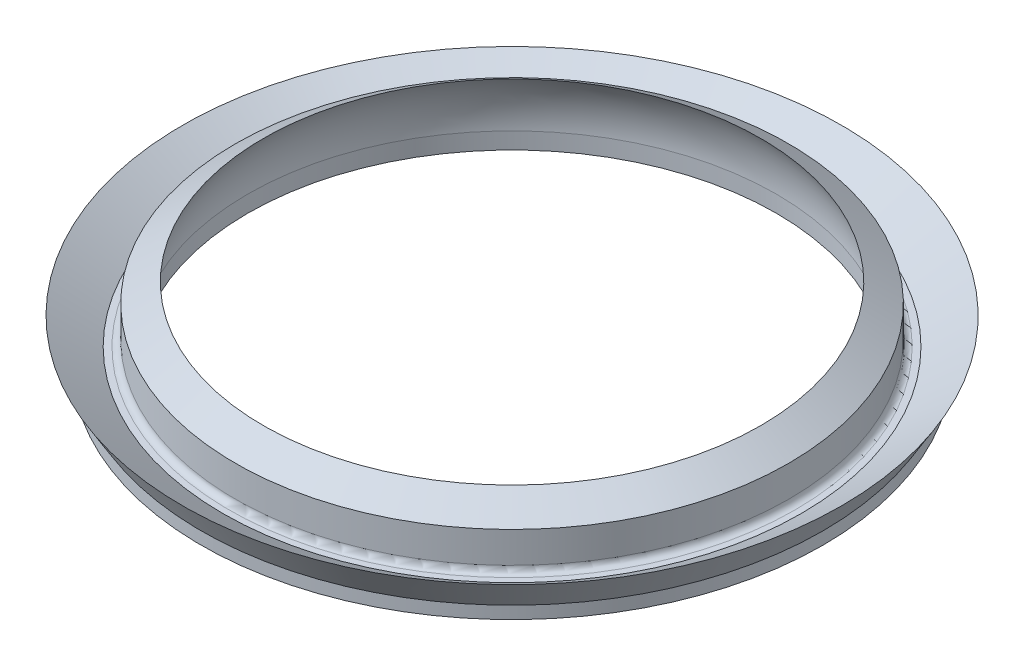
SolidWorks part; units mm, degrees
material "硅橡胶"
ref_plane "前视基准面" through (0, 0, 0) normal (0, 0, 1) x (1, 0, 0)
ref_plane "上视基准面" through (0, 0, 0) normal (0, 1, 0) x (1, 0, 0)
ref_plane "右视基准面" through (0, 0, 0) normal (1, 0, 0) x (0, 0, -1)
sketch "草图1" plane through (0, 0, 0) normal (0, 0, 1) x (1, 0, 0)
  line L0 (0, -5.5) -> (0, 5.5) construction
  line L1 (42.5, -6.1699) -> (49.9955, -6.1699)
  line L2 (49.9955, -6.1699) -> (49.9955, -4.1699)
  line L3 (46.5, -3.5) -> (45.5, -3.5)
  line L4 (42.5, -3.5) -> (42.5, -6.1699)
  line L5 (0, 0.8301) -> (53, 0.8301) construction
  line L6 (53, 0.8301) -> (49.9955, -4.1699)
  line L7 (46.5, -3.5) -> (46.5, -0.7454) construction
  line L8 (46.5, -3.5) -> (53, 0.8301)
  line L9 (44.5, 2.5) -> (44.5, -2.5)
  line L11 (44.5, 2.5) -> (40, 5.5)
  arc A0 (40, 5.5) -> (42.5, -3.5) centre (27.5156, -2.8151) cw
  arc A1 (44.5, -2.5) -> (45.5, -3.5) centre (45.5, -2.5) ccw
  point P4 (0, 0)
  dimension "D12" = 15
  dimension "D14" = 1
  dimension "D1" = 11
  dimension "D2" = 50
  dimension "D3" = 2
  dimension "D4" = 42.5
  dimension "D6" = 7
  dimension "D7" = 53
  dimension "D8" = 4
  dimension "D9" = 7.8102
  dimension "D10" = 3
  dimension "D11" = 40
  dimension "D13" = 5
  dimension "D15" = 1
  dimension "D16" = 1
  dimension "D17" = 90
revolve "旋转1" add sketch "草图1" angle 360 about L0
